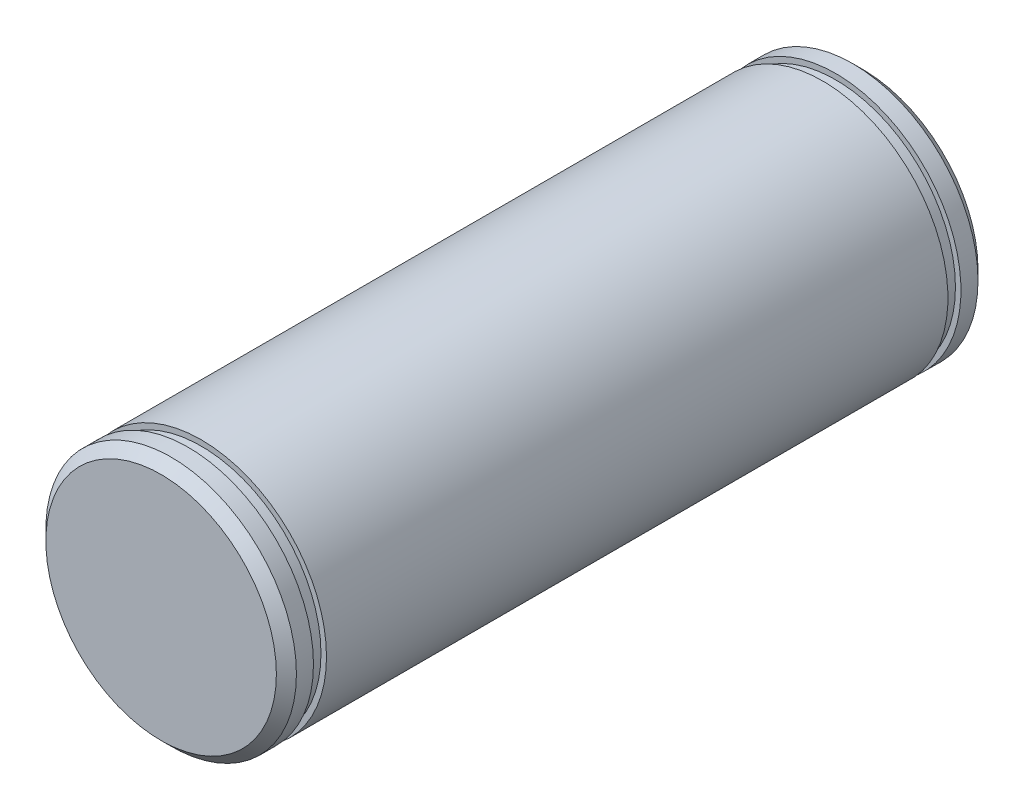
from build123d import *

# Parameters (mm, degrees)
SKETCH_1_R      = 12.5
EXTRUDE_1_DEPTH = 35
SKETCH_3_W      = 1.3
SKETCH_3_H      = 0.55
SKETCH_31_W     = 1.3
SKETCH_31_H     = 0.55
CHAMFER_1_SIZE  = 1


with BuildPart() as part:
    # 草图1 → 凸台-拉伸1 (new, symmetric)
    with BuildSketch(Plane.XY):
        Circle(SKETCH_1_R)
    extrude(amount=EXTRUDE_1_DEPTH, both=True)

    # 草图3 → 切除-旋转1 (revolve, cut)
    with BuildSketch(Plane(origin=(-100, 0, -35), x_dir=(0, 0, 1), z_dir=(0, 1, 0))):
        with Locations((3.35, 87.775)):
            Rectangle(SKETCH_3_W, SKETCH_3_H)
    revolve(axis=Axis((0, 0, -35), (0, 0, 1)), mode=Mode.SUBTRACT)

    # 草图31 → 切除-旋转11 (revolve, cut)
    with BuildSketch(Plane(origin=(100, 0, 35), x_dir=(0, 0, -1), z_dir=(0, 1, 0)), mode=Mode.PRIVATE) as cut_revolve_11_sk:
        with Locations((3.35, 87.775)):
            Rectangle(SKETCH_31_W, SKETCH_31_H)
    revolve(cut_revolve_11_sk.sketch.rotate(Axis((0, 0, 35), (0, 0, -1)), 180), axis=Axis((0, 0, 35), (0, 0, -1)), mode=Mode.SUBTRACT)

    # 倒角1
    chamfer_1_edges = [part.edges().sort_by_distance(p)[0] for p in [
        (-12.5, 0, -35),
        (-12.5, 0, 35),
    ]]
    chamfer(chamfer_1_edges, length=CHAMFER_1_SIZE)


solid = part.part
